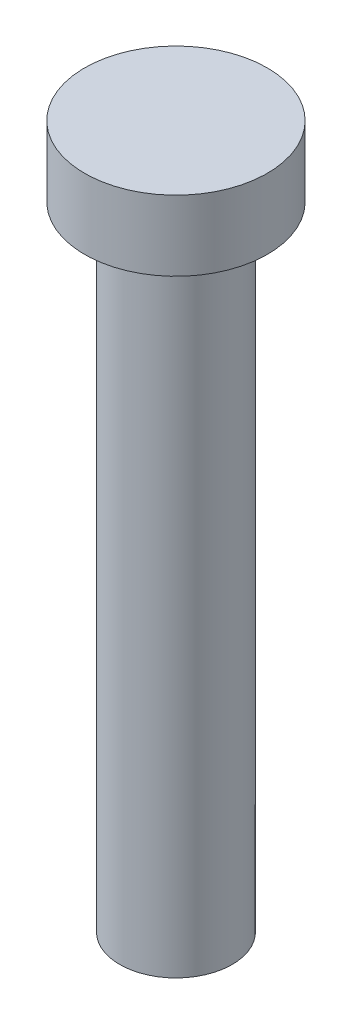
from build123d import *


with BuildPart() as part:
    # Sketch1 → Revolve1 (revolve)
    with BuildSketch(Plane.XY, mode=Mode.PRIVATE) as revolve1_sk:
        Polygon((0, 0), (0, 50), (6.5, 50), (6.5, 45), (4, 45), (4, 0), align=None)
    revolve(revolve1_sk.sketch.rotate(Axis((0, 0, 0), (0, 1, 0)), 90), axis=Axis((0, 0, 0), (0, 1, 0)))


solid = part.part
